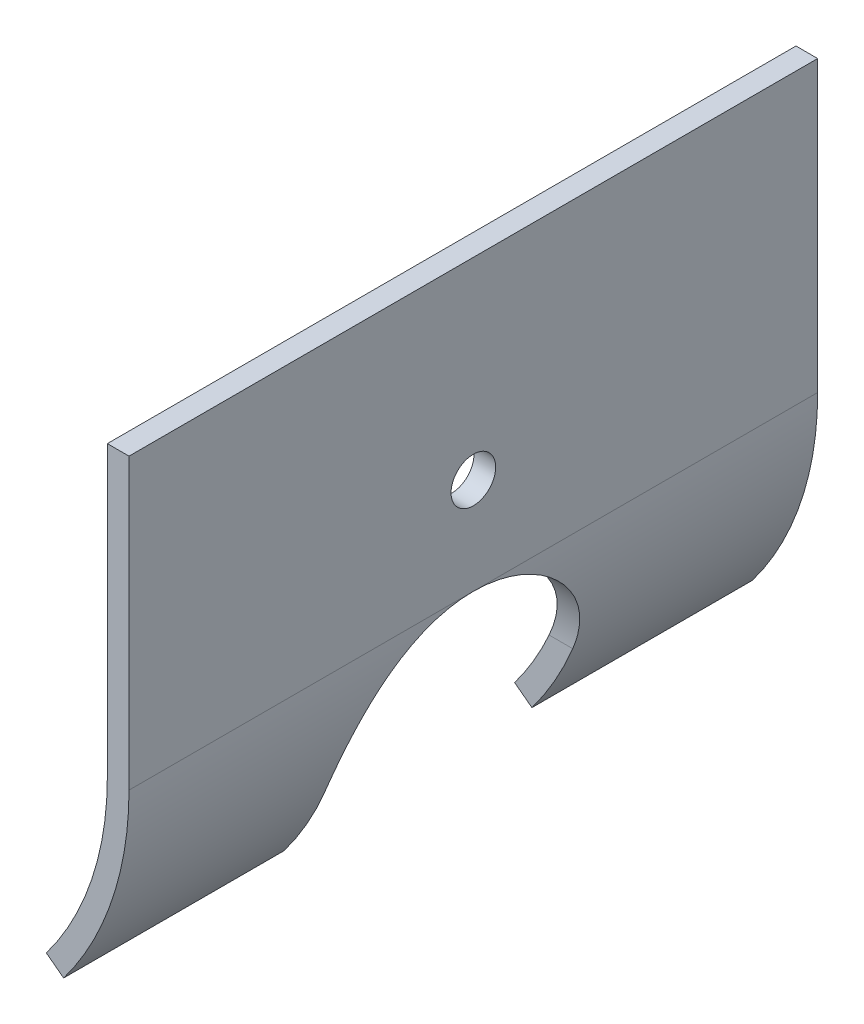
from build123d import *

# Parameters (mm, degrees)
BOSS_EXTRUDE1_DEPTH = 158.75
SKETCH4_R           = 10.287
CUT_EXTRUDE1_DEPTH  = 184.15


with BuildPart() as part:
    # Sketch1 → Boss-Extrude1 (new, symmetric)
    with BuildSketch(Plane.XY):
        with BuildLine():
            Line((-10, 88.9), (0, 88.9))
            Line((0, 88.9), (0, -44.45))
            ThreePointArc((0, -44.45), (-7.735948816, -91.950507064), (-30.144264146, -134.541708966))
            Line((-30.144264146, -134.541708966), (-38.130619246, -128.523558734))
            ThreePointArc((-38.130619246, -128.523558734), (-17.219185368, -88.7774605), (-10, -44.45))
            Line((-10, -44.45), (-10, 88.9))
        make_face()
    extrude(amount=BOSS_EXTRUDE1_DEPTH, both=True)

    # Sketch4 → Cut-Extrude1 (cut, symmetric)
    with BuildSketch(Plane(origin=(0, 0, 0), x_dir=(0, 0, -1), z_dir=(1, 0, 0))):
        Circle(SKETCH4_R)
        with BuildLine():
            Line((-57.15, -101.6), (-57.15, -134.541708966))
            Line((-57.15, -134.541708966), (57.15, -134.541708966))
            Line((57.15, -134.541708966), (57.15, -101.6))
            ThreePointArc((57.15, -101.6), (0, -44.45), (-57.15, -101.6))
        make_face()
    extrude(amount=CUT_EXTRUDE1_DEPTH, both=True, mode=Mode.SUBTRACT)


solid = part.part
